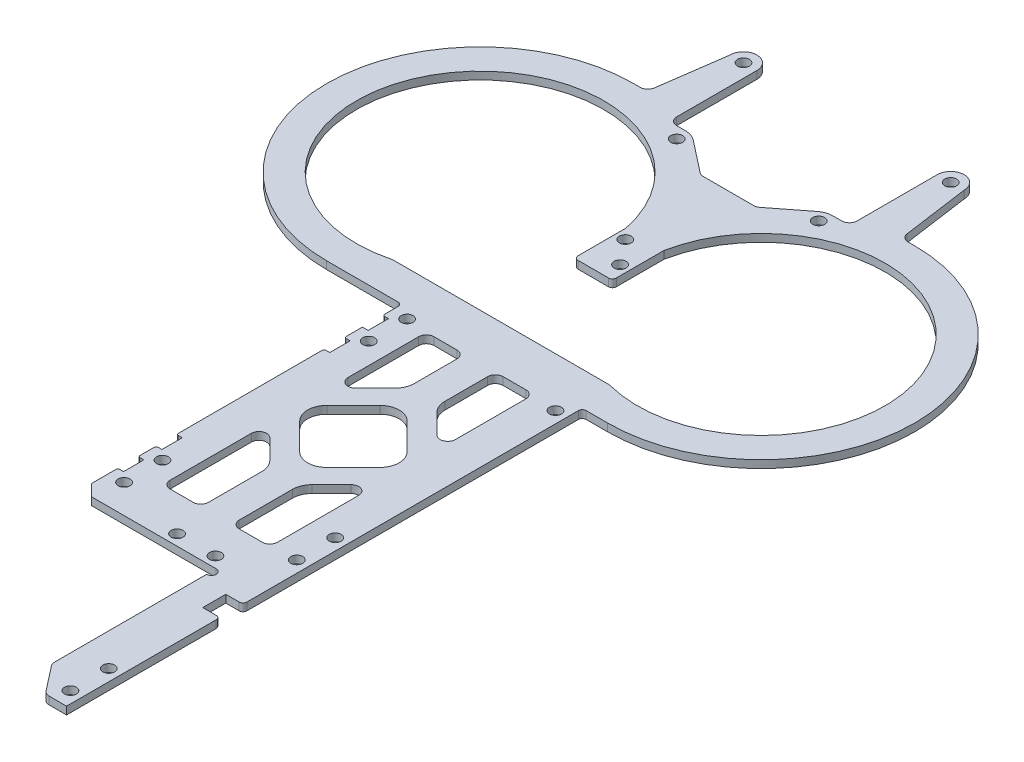
SolidWorks part; units mm, degrees
material "Thornel Mat VMA"
ref_plane "前视基准面" through (0, 0, 0) normal (0, 0, 1) x (1, 0, 0)
ref_plane "上视基准面" through (0, 0, 0) normal (0, 1, 0) x (1, 0, 0)
ref_plane "右视基准面" through (0, 0, 0) normal (1, 0, 0) x (0, 0, -1)
other "Configuration Table"
sketch "草图1" plane through (0, 0, 0) normal (0, 1, 0) x (1, 0, 0)
  line L0 (0, 0) -> (3.7241, 0) construction
  line L1 (0, 0) -> (0, 17.4538) construction
  line L2 (17.5, 36.1) -> (23.5, 36.1)
  line L4 (17.5, 36.1) -> (7.2605, 28.1)
  line L5 (7.2605, 28.1) -> (-7.2605, 28.1)
  line L7 (-17.5, 36.1) -> (-23.5, 36.1)
  line L8 (-17.5, 36.1) -> (-7.2605, 28.1)
  line L9 (36.625, -40) -> (30, -40)
  line L10 (-36.625, -40) -> (-17, -40)
  line L11 (-17, -40) -> (-17, -123.9)
  line L12 (30, -40) -> (30, -123.9)
  line L13 (-13, -42.65) -> (-13, -52.65) construction
  line L15 (-17, -123.9) -> (18.5, -123.9)
  line L16 (30, -123.9) -> (30, -174.4)
  line L17 (30, -174.4) -> (24.5, -174.4)
  line L18 (24.5, -174.4) -> (18.5, -166.7204)
  line L19 (18.5, -166.7204) -> (18.5, -123.9)
  line L20 (-5, 6.3184) -> (-5, -7.15)
  line L21 (-5, -7.15) -> (5, -7.15)
  line L22 (5, -7.15) -> (5, 6.3184)
  line L23 (-28.274, -31.15) -> (28.274, -31.15)
  line L24 (-23.5, 59) -> (-23.5, 36.1)
  line L28 (-36.625, 40) -> (-33.1703, 40)
  line L29 (-33.1703, 40) -> (-30.5, 59)
  line L30 (23.5, 59) -> (23.5, 36.1)
  line L31 (33.1703, 40) -> (30.5, 59)
  line L32 (33.1703, 40) -> (36.625, 40)
  arc A0 (28.274, -31.15) -> (5, 6.3184) centre (36.625, 0) ccw
  circle A1 centre (18.5, 33.1) radius 1.55
  arc A2 (36.625, -40) -> (36.625, 40) centre (36.625, 0) ccw
  arc A3 (-28.274, -31.15) -> (-5, 6.3184) centre (-36.625, 0) cw
  arc A4 (-36.625, -40) -> (-36.625, 40) centre (-36.625, 0) cw
  circle A5 centre (-18.5, 33.1) radius 1.55
  circle A6 centre (27, -44) radius 1.55
  circle A7 centre (27, -101.4) radius 1.55
  circle A8 centre (27, -111.4) radius 1.55
  circle A9 centre (-13, -42.65) radius 1.55
  circle A10 centre (-13, -52.65) radius 1.55
  circle A11 centre (-13, -106.4) radius 1.55
  circle A12 centre (-13, -116.4) radius 1.55
  circle A13 centre (5.5, -121.1) radius 1.55
  circle A14 centre (15.5, -121.1) radius 1.55
  circle A15 centre (27, -160.4) radius 1.55
  circle A16 centre (27, -170.4) radius 1.55
  circle A17 centre (-2.5, 3.7) radius 1.55
  circle A18 centre (2.5, -2.65) radius 1.55
  circle A19 centre (-27, 59) radius 1.55
  arc A20 (-23.5, 59) -> (-30.5, 59) centre (-27, 59) ccw
  circle A21 centre (27, 59) radius 1.55
  arc A22 (23.5, 59) -> (30.5, 59) centre (27, 59) cw
  point P25 (0, 28.1)
  dimension "D1" = 64.5
  dimension "D2" = 36.625
  dimension "D4" = 3.1
  dimension "D5" = 33.1
  dimension "D8" = 3
  dimension "D9" = 40
  dimension "D13" = 3.1
  dimension "D14" = 8.5
  dimension "D16" = 10
  dimension "D17" = 57.4
  dimension "D18" = 31.5
  dimension "D21" = 10
  dimension "D22" = 53.75
  dimension "D23" = 4
  dimension "D24" = 4.7
  dimension "D25" = 10
  dimension "D26" = 2.8
  dimension "D27" = 18.5
  dimension "D31" = 10
  dimension "D32" = 4
  dimension "D33" = 29.4
  dimension "D34" = 16
  dimension "D35" = 35.75
  dimension "D36" = 16
  dimension "D40" = 8.5
  dimension "D41" = 25.9
  dimension "D42" = 7
  dimension "D3" = 18.5
  dimension "D6" = 5
  dimension "D7" = 1
  dimension "D10" = 8
  dimension "D11" = 52
  dimension "D12" = 44
  dimension "D15" = 3
  dimension "D19" = 10
  dimension "D20" = 1.35
  dimension "D28" = 11.5
  dimension "D29" = 5.5
  dimension "D30" = 50.5
  dimension "D37" = 2.5
  dimension "D38" = 24
  dimension "D39" = 4.5
  dimension "D43" = 8
extrude "凸台-拉伸1" add sketch "草图1" along normal blind 2
sketch "草图3" plane through (0, 2, 0) normal (0, 1, 0) x (1, 0, 0)
  line L0 (-17, -40) -> (-17, -123.9) construction
  line L1 (-17, -45) -> (-15.5, -45)
  line L2 (-17, -45) -> (-17, -50.3)
  line L3 (-17, -50.3) -> (-15.5, -50.3)
  line L4 (-15.5, -45) -> (-15.5, -50.3)
  line L5 (-13, -42.65) -> (-13, -52.65) construction
  line L6 (-17, -55) -> (-15.5, -55)
  line L7 (-17, -55) -> (-17, -60.3)
  line L8 (-17, -60.3) -> (-15.5, -60.3)
  line L9 (-15.5, -55) -> (-15.5, -60.3)
  line L10 (-17, -47.65) -> (-15.5, -47.65) construction
  line L11 (-17, -98.75) -> (-15.5, -98.75)
  line L12 (-17, -98.75) -> (-17, -104.05)
  line L13 (-15.5, -98.75) -> (-15.5, -104.05)
  line L14 (-17, -104.05) -> (-15.5, -104.05)
  line L15 (-17, -108.75) -> (-15.5, -108.75)
  line L16 (-17, -108.75) -> (-17, -114.05)
  line L17 (-15.5, -108.75) -> (-15.5, -114.05)
  line L18 (-17, -114.05) -> (-15.5, -114.05)
  line L19 (-17, -101.4) -> (-15.5, -101.4) construction
  line L20 (18.5, -123.9) -> (18.5, -166.7204) construction
  line L21 (30, -174.4) -> (30, -40) construction
  line L22 (30, -128.4) -> (25.5, -128.4)
  line L23 (30, -128.4) -> (30, -134.4)
  line L24 (30, -134.4) -> (25.5, -134.4)
  line L25 (25.5, -128.4) -> (25.5, -134.4)
  line L26 (6.5, -182.9013) -> (6.5, 59.3678) construction
  line L27 (6.5, -90.15) -> (20.5, -76.15)
  line L28 (6.5, -90.15) -> (-7.5, -76.15)
  line L29 (20.5, -76.15) -> (6.5, -62.15)
  line L30 (-7.5, -76.15) -> (6.5, -62.15)
  line L31 (-7.5, -68.3718) -> (2.5, -58.3718)
  line L32 (2.5, -58.3718) -> (2.5, -43.15)
  line L33 (2.5, -43.15) -> (-7.5, -43.15)
  line L34 (-7.5, -43.15) -> (-7.5, -68.3718)
  line L35 (-28.274, -31.15) -> (28.274, -31.15) construction
  line L37 (-7.5, -83.9282) -> (-7.5, -111.9)
  line L38 (-7.5, -111.9) -> (2.5, -111.9)
  line L39 (2.5, -111.9) -> (2.5, -93.9282)
  line L40 (2.5, -93.9282) -> (-7.5, -83.9282)
  line L41 (-17, -123.9) -> (18.5, -123.9) construction
  line L42 (10.5, -93.9282) -> (20.5, -83.9282)
  line L43 (10.5, -111.9) -> (10.5, -93.9282)
  line L44 (20.5, -111.9) -> (10.5, -111.9)
  line L45 (20.5, -83.9282) -> (20.5, -111.9)
  line L46 (20.5, -43.15) -> (20.5, -68.3718)
  line L47 (10.5, -43.15) -> (20.5, -43.15)
  line L48 (10.5, -58.3718) -> (10.5, -43.15)
  line L49 (20.5, -68.3718) -> (10.5, -58.3718)
  circle A1 centre (-13, -42.65) radius 1.55 construction
  circle A2 centre (-13, -106.4) radius 1.55 construction
  circle A3 centre (18.5, -125.15) radius 1.25
  circle A4 centre (27, -111.4) radius 1.55 construction
  dimension "D6" = 5
  dimension "D7" = 2.5
  dimension "D1" = 1.5
  dimension "D2" = 5
  dimension "D3" = 5.3
  dimension "D4" = 10
  dimension "D8" = 4.5
  dimension "D9" = 6
  dimension "D10" = 17
  dimension "D11" = 23.5
  dimension "D12" = 28
  dimension "D13" = 4
  dimension "D14" = 12
  dimension "D15" = 5.5
  dimension "D16" = 45
  dimension "D17" = 12
  dimension "D18" = 5.5
  dimension "D5" = 2
extrude "切除-拉伸1" cut sketch "草图3" against normal blind 3.2
chamfer "倒角1" distance 3 angle 45 1 edges at (-17, 1, 123.9)
fillet "圆角1" radius 2 22 edges at (7.2605, 1, -28.1) (-7.2605, 1, -28.1) (28.274, 1, 31.15) (-28.274, 1, 31.15) (24.5, 1, 174.4) (18.5, 1, 166.7204) (33.1703, 1, -40) (23.5, 1, -36.1) (-23.5, 1, -36.1) (-33.1703, 1, -40) (-7.5, 1, 111.9) (-7.5, 1, 83.9282) (2.5, 1, 111.9) (20.5, 1, 111.9) (10.5, 1, 111.9) (20.5, 1, 83.9282) (20.5, 1, 68.3718) (10.5, 1, 43.15) (20.5, 1, 43.15) (-7.5, 1, 43.15) (2.5, 1, 43.15) (-7.5, 1, 68.3718)
fillet "圆角2" radius 5 10 edges at (17.5, 1, -36.1) (-17.5, 1, -36.1) (20.5, 1, 76.15) (6.5, 1, 90.15) (-7.5, 1, 76.15) (10.5, 1, 93.9282) (2.5, 1, 93.9282) (10.5, 1, 58.3718) (2.5, 1, 58.3718) (6.5, 1, 62.15)
fillet "圆角3" radius 0.5 8 edges at (-17, 1, 114.05) (-17, 1, 108.75) (-17, 1, 104.05) (-17, 1, 98.75) (-17, 1, 60.3) (-17, 1, 55) (-16.25, 0, 50.3) (-17, 1, 45)
fillet "圆角4" radius 1 8 edges at (30, 1, 134.4) (30, 1, 128.4) (-5, 1, -6.3184) (5, 1, -6.3184) (5, 1, 7.15) (-5, 1, 7.15) (30, 1, 40) (-17, 1, 40)
sketch "草图4" [suppressed] plane through (0, 2, 0) normal (0, 1, 0) x (1, 0, 0)
  line L12 (18.5, -43.15) -> (12.5, -43.15)
  line L13 (20.5, -63.5434) -> (20.5, -45.15)
  line L14 (11.9645, -59.8363) -> (17.0858, -64.9576)
  line L15 (10.5, -45.15) -> (10.5, -56.3008)
  line L16 (18.5, -43.15) -> (12.5, -43.15)
  line L17 (20.5, -63.5434) -> (20.5, -45.15)
  line L18 (11.9645, -59.8363) -> (17.0858, -64.9576)
  line L19 (10.5, -45.15) -> (10.5, -56.3008)
  line L20 (2.5, -109.9) -> (2.5, -95.9992)
  line L21 (-5.5, -111.9) -> (0.5, -111.9)
  line L22 (-7.5, -88.7566) -> (-7.5, -109.9)
  line L23 (1.0355, -92.4637) -> (-4.0858, -87.3424)
  line L24 (2.5, -109.9) -> (2.5, -95.9992)
  line L25 (-5.5, -111.9) -> (0.5, -111.9)
  line L26 (-7.5, -88.7566) -> (-7.5, -109.9)
  line L27 (1.0355, -92.4637) -> (-4.0858, -87.3424)
  line L28 (10.5, -95.9992) -> (10.5, -109.9)
  line L29 (17.0858, -87.3424) -> (11.9645, -92.4637)
  line L30 (20.5, -109.9) -> (20.5, -88.7566)
  line L31 (12.5, -111.9) -> (18.5, -111.9)
  line L32 (10.5, -95.9992) -> (10.5, -109.9)
  line L33 (17.0858, -87.3424) -> (11.9645, -92.4637)
  line L34 (20.5, -109.9) -> (20.5, -88.7566)
  line L35 (12.5, -111.9) -> (18.5, -111.9)
  line L36 (0.5, -43.15) -> (-5.5, -43.15)
  line L37 (2.5, -56.3008) -> (2.5, -45.15)
  line L38 (-4.0858, -64.9576) -> (1.0355, -59.8363)
  line L39 (-7.5, -45.15) -> (-7.5, -63.5434)
  line L40 (0.5, -43.15) -> (-5.5, -43.15)
  line L41 (2.5, -56.3008) -> (2.5, -45.15)
  line L42 (-4.0858, -64.9576) -> (1.0355, -59.8363)
  line L43 (-7.5, -45.15) -> (-7.5, -63.5434)
  line L44 (-3.9645, -79.6855) -> (2.9645, -86.6145)
  line L45 (2.9645, -65.6855) -> (-3.9645, -72.6145)
  line L46 (16.9645, -72.6145) -> (10.0355, -65.6855)
  line L47 (10.0355, -86.6145) -> (16.9645, -79.6855)
  line L48 (-3.9645, -79.6855) -> (2.9645, -86.6145)
  line L49 (2.9645, -65.6855) -> (-3.9645, -72.6145)
  line L50 (16.9645, -72.6145) -> (10.0355, -65.6855)
  line L51 (10.0355, -86.6145) -> (16.9645, -79.6855)
  arc A4 (20.5, -45.15) -> (18.5, -43.15) centre (18.5, -45.15) ccw
  arc A5 (17.0858, -64.9576) -> (20.5, -63.5434) centre (18.5, -63.5434) ccw
  arc A6 (10.5, -56.3008) -> (11.9645, -59.8363) centre (15.5, -56.3008) ccw
  arc A7 (12.5, -43.15) -> (10.5, -45.15) centre (12.5, -45.15) ccw
  arc A24 (20.5, -45.15) -> (18.5, -43.15) centre (18.5, -45.15) ccw
  arc A25 (17.0858, -64.9576) -> (20.5, -63.5434) centre (18.5, -63.5434) ccw
  arc A26 (10.5, -56.3008) -> (11.9645, -59.8363) centre (15.5, -56.3008) ccw
  arc A27 (12.5, -43.15) -> (10.5, -45.15) centre (12.5, -45.15) ccw
  arc A28 (0.5, -111.9) -> (2.5, -109.9) centre (0.5, -109.9) ccw
  arc A29 (-7.5, -109.9) -> (-5.5, -111.9) centre (-5.5, -109.9) ccw
  arc A30 (-4.0858, -87.3424) -> (-7.5, -88.7566) centre (-5.5, -88.7566) ccw
  arc A31 (2.5, -95.9992) -> (1.0355, -92.4637) centre (-2.5, -95.9992) ccw
  arc A32 (0.5, -111.9) -> (2.5, -109.9) centre (0.5, -109.9) ccw
  arc A33 (-7.5, -109.9) -> (-5.5, -111.9) centre (-5.5, -109.9) ccw
  arc A34 (-4.0858, -87.3424) -> (-7.5, -88.7566) centre (-5.5, -88.7566) ccw
  arc A35 (2.5, -95.9992) -> (1.0355, -92.4637) centre (-2.5, -95.9992) ccw
  arc A36 (11.9645, -92.4637) -> (10.5, -95.9992) centre (15.5, -95.9992) ccw
  arc A37 (20.5, -88.7566) -> (17.0858, -87.3424) centre (18.5, -88.7566) ccw
  arc A38 (18.5, -111.9) -> (20.5, -109.9) centre (18.5, -109.9) ccw
  arc A39 (10.5, -109.9) -> (12.5, -111.9) centre (12.5, -109.9) ccw
  arc A40 (11.9645, -92.4637) -> (10.5, -95.9992) centre (15.5, -95.9992) ccw
  arc A41 (20.5, -88.7566) -> (17.0858, -87.3424) centre (18.5, -88.7566) ccw
  arc A42 (18.5, -111.9) -> (20.5, -109.9) centre (18.5, -109.9) ccw
  arc A43 (10.5, -109.9) -> (12.5, -111.9) centre (12.5, -109.9) ccw
  arc A44 (2.5, -45.15) -> (0.5, -43.15) centre (0.5, -45.15) ccw
  arc A45 (1.0355, -59.8363) -> (2.5, -56.3008) centre (-2.5, -56.3008) ccw
  arc A46 (-7.5, -63.5434) -> (-4.0858, -64.9576) centre (-5.5, -63.5434) ccw
  arc A47 (-5.5, -43.15) -> (-7.5, -45.15) centre (-5.5, -45.15) ccw
  arc A48 (2.5, -45.15) -> (0.5, -43.15) centre (0.5, -45.15) ccw
  arc A49 (1.0355, -59.8363) -> (2.5, -56.3008) centre (-2.5, -56.3008) ccw
  arc A50 (-7.5, -63.5434) -> (-4.0858, -64.9576) centre (-5.5, -63.5434) ccw
  arc A51 (-5.5, -43.15) -> (-7.5, -45.15) centre (-5.5, -45.15) ccw
  arc A68 (-3.9645, -72.6145) -> (-3.9645, -79.6855) centre (-0.4289, -76.15) ccw
  arc A69 (10.0355, -65.6855) -> (2.9645, -65.6855) centre (6.5, -69.2211) ccw
  arc A70 (16.9645, -79.6855) -> (16.9645, -72.6145) centre (13.4289, -76.15) ccw
  arc A71 (2.9645, -86.6145) -> (10.0355, -86.6145) centre (6.5, -83.0789) ccw
  arc A72 (-3.9645, -72.6145) -> (-3.9645, -79.6855) centre (-0.4289, -76.15) ccw
  arc A73 (10.0355, -65.6855) -> (2.9645, -65.6855) centre (6.5, -69.2211) ccw
  arc A74 (16.9645, -79.6855) -> (16.9645, -72.6145) centre (13.4289, -76.15) ccw
  arc A75 (2.9645, -86.6145) -> (10.0355, -86.6145) centre (6.5, -83.0789) ccw
  dimension "D2" = 0
  dimension "D3" = 0
  dimension "D4" = 0
  dimension "D5" = 0
  dimension "D14" = 0
extrude "凸台-拉伸3" [suppressed] add sketch "草图4" against normal up to surface (2 mm away)
sketch "草图5" plane through (0, 2, 0) normal (0, 1, 0) x (1, 0, 0)
  line L0 (-486.9738, 279.8984) -> (-60.3071, 279.8984) construction
  line L1 (7.0174, -100.5345) -> (9.787, -105.2631)
  line L2 (9.787, -105.2631) -> (12.5757, -98.2412)
  line L3 (18.5687, -91.6177) -> (22.6894, -75.4728)
  line L4 (-7.6413, -52.2351) -> (14.7136, -81.1684)
  line L5 (14.7136, -78.7946) -> (12.2593, -74.8262)
  line L6 (6.2638, -67.3993) -> (9.1096, -71.2291)
  spline S0 degree 2 poles (-7.6413, -52.2351) (1.4884, -65.3548) (6.0041, -80.7419) knots 0 0 0 1 1 1
  spline S1 degree 2 poles (6.0041, -80.7419) (7.4852, -90.5987) (7.0174, -100.5345) knots 0 0 0 1 1 1
  spline S2 degree 2 poles (12.5757, -98.2412) (13.4758, -92.6508) (18.5687, -91.6177) knots 0 0 0 1 1 1
  spline S3 degree 2 poles (22.6894, -75.4728) (24.0018, -69.3743) (23.4324, -63.1785) knots 0 0 0 1 1 1
  spline S4 degree 2 poles (14.7136, -81.1684) (16.4783, -83.3782) (18.5687, -80.7419) knots 0 0 0 1 1 1
  spline S5 degree 2 poles (23.4324, -63.1785) (22.5559, -72.4541) (18.5687, -80.7419) knots 0 0 0 1 1 1
  spline S6 degree 2 poles (12.2593, -74.8262) (13.8473, -68.3543) (14.2324, -61.6987) knots 0 0 0 1 1 1
  spline S7 degree 2 poles (14.2324, -61.6987) (15.753, -70.2244) (14.7136, -78.7946) knots 0 0 0 1 1 1
  spline S8 degree 2 poles (5.1298, -57.926) (6.1878, -62.6068) (6.2638, -67.3993) knots 0 0 0 1 1 1
  spline S9 degree 2 poles (5.1298, -57.926) (8.4659, -64.2392) (9.1096, -71.2291) knots 0 0 0 1 1 1
extrude "切除-拉伸2" [suppressed] cut sketch "草图5" against normal through all
